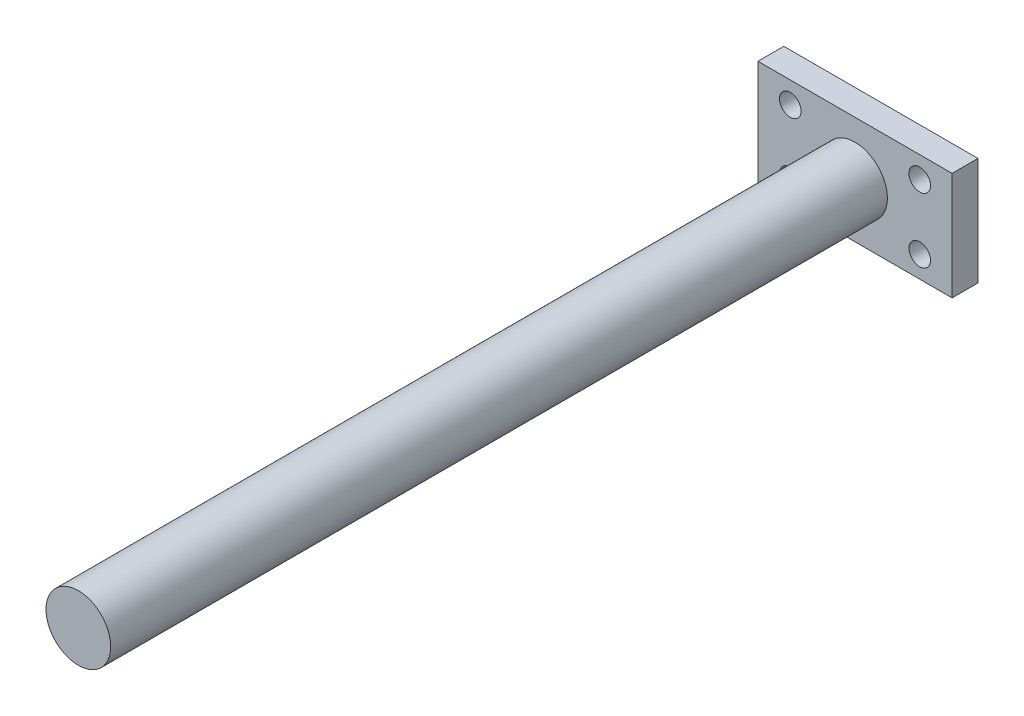
from build123d import *

# Parameters (mm, degrees)
SKETCH1_W           = 90
SKETCH1_H           = 50
SKETCH1_R           = 5
BOSS_EXTRUDE1_DEPTH = 12
SKETCH2_R           = 15
BOSS_EXTRUDE2_DEPTH = 360


with BuildPart() as part:
    # Sketch1 → Boss-Extrude1 (new body)
    with BuildSketch(Plane.XY):
        Rectangle(SKETCH1_W, SKETCH1_H)
        with Locations((-30, 15)):
            Circle(SKETCH1_R, mode=Mode.SUBTRACT)
        with Locations((-30, -15)):
            Circle(SKETCH1_R, mode=Mode.SUBTRACT)
        with Locations((30, -15)):
            Circle(SKETCH1_R, mode=Mode.SUBTRACT)
        with Locations((30, 15)):
            Circle(SKETCH1_R, mode=Mode.SUBTRACT)
    extrude(amount=BOSS_EXTRUDE1_DEPTH)

    # Sketch2 → Boss-Extrude2 (add)
    with BuildSketch(Plane.XY.offset(12)):
        with Locations(Location((0, 0, 0), (0, 0, 180))):
            Circle(SKETCH2_R)
    extrude(amount=BOSS_EXTRUDE2_DEPTH)


solid = part.part
